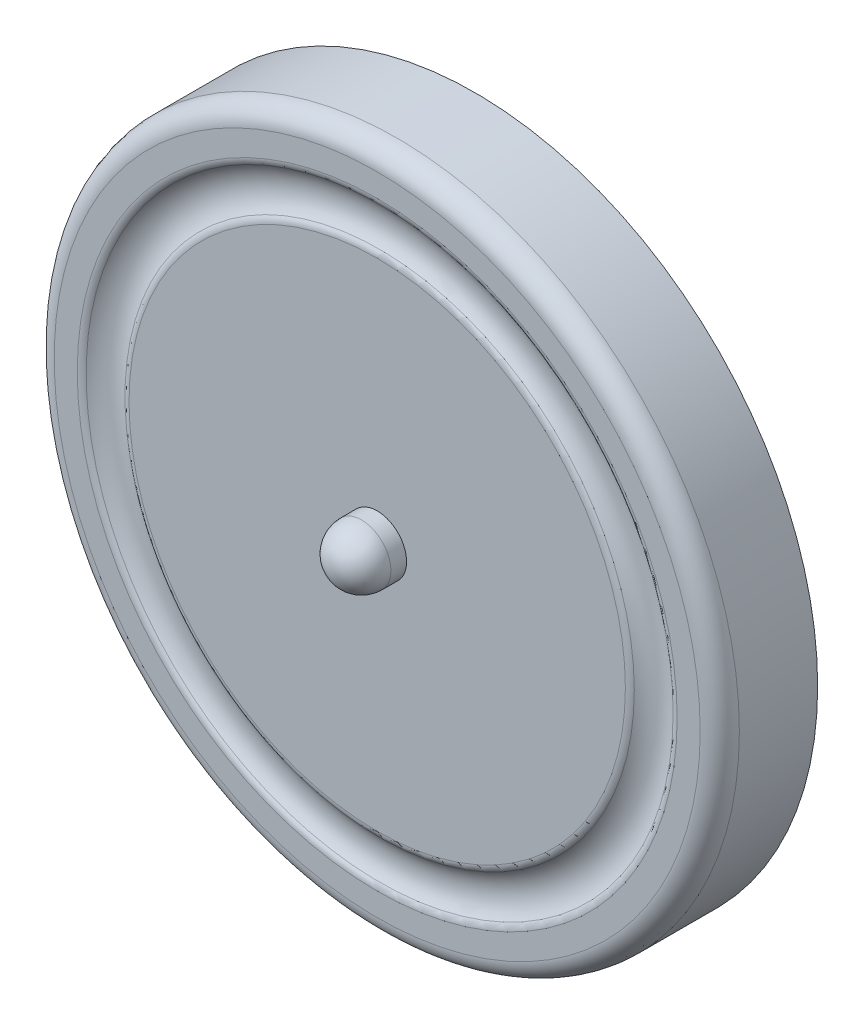
SolidWorks part; units mm, degrees
material "1.4000 (X6Cr13)"
ref_plane "Front Plane" through (0, 0, 0) normal (0, 0, 1) x (1, 0, 0)
ref_plane "Top Plane" through (0, 0, 0) normal (0, 1, 0) x (1, 0, 0)
ref_plane "Right Plane" through (0, 0, 0) normal (1, 0, 0) x (0, 0, -1)
sketch "Sketch1" plane through (0, 0, 0) normal (0, 0, 1) x (1, 0, 0)
  circle A0 centre (-121.5312, 115.619) radius 17.5
  arc A1 (-138.8054, 118.4212) -> (-107.4951, 105.1673) centre (-121.5312, 115.619) ccw construction
extrude "Boss-Extrude1" add sketch "Sketch1" along normal blind 5
ref_plane "Plane4" through (-144.5684, 61.1971, 0) normal (0.9209, -0.3898, 0) x (-0.3898, -0.9209, 0)
sketch "Sketch2" plane through (-144.5684, 61.1971, 0) normal (0.9209, -0.3898, 0) x (-0.3898, -0.9209, 0)
  line L0 (-59.097, -5.8768) -> (-59.097, 1.1833) construction
  line L1 (-59.097, -5) -> (-59.097, 0) construction
  line L2 (-59.097, -7.5) -> (-59.097, 10.5) construction
  line L3 (-41.597, 0) -> (-76.597, 0) construction
  line L4 (-59.097, 0) -> (-53.597, 0)
  line L5 (-59.097, 0) -> (-59.097, -2)
  line L6 (-59.097, -2) -> (-54.597, -2)
  line L7 (-53.597, 0) -> (-53.597, -1)
  arc A1 (-53.597, -1) -> (-54.597, -2) centre (-54.597, -1) cw
  point P14 (-53.597, -2)
  dimension "D3" = 1
  dimension "D1" = 11
  dimension "D2" = 2
revolve "Cut-Revolve1" cut sketch "Sketch2" angle 360 about L0
sketch "Sketch4" plane through (-144.5684, 61.1971, 0) normal (0.9209, -0.3898, 0) x (-0.3898, -0.9209, 0)
  line L0 (-59.097, -5) -> (-59.097, -2) construction
  line L1 (-76.597, -5) -> (-41.597, -5) construction
  line L2 (-59.097, 2.1177) -> (-59.097, -7.2354) construction
  line L3 (-59.097, 3.5) -> (-59.097, 2.5) construction
  line L4 (-54.597, -2) -> (-63.597, -2) construction
  line L7 (-59.097, -2) -> (-59.097, 3)
  arc A0 (-59.097, -2) -> (-59.097, 3) centre (-59.097, 0.5) ccw construction
  arc A1 (-59.097, -2) -> (-59.097, 3) centre (-59.097, 0.5) ccw
  dimension "D1" = 5
  dimension "D2" = 2.5
revolve "Revolve1" add sketch "Sketch4" angle 360 about L0
ref_plane "Plane5" through (0, 115.619, 0) normal (0, 1, 0) x (0, 0, 1)
sketch "Sketch5" plane through (0, 115.619, 0) normal (0, 1, 0) x (0, 0, 1)
  line L1 (5, -121.5312) -> (0, -121.5312) construction
  line L2 (5, -139.0312) -> (5, -104.0312) construction
  circle A0 centre (6, -107.5312) radius 1.5
  dimension "D2" = 3
  dimension "D1" = 14
  dimension "D3" = 1
revolve "Cut-Revolve2" cut sketch "Sketch5" angle 360 about axis through (-121.5312, 115.619, 5) along (0, 0, -1)
fillet "Fillet1" radius 1 1 edges at (-104.0312, 115.619, 5)
fillet "Fillet2" radius 0.5 2 edges at (-106.4131, 115.619, 5) (-134.4131, 115.619, 5)
sketch "Sketch6" plane through (0, 115.619, 0) normal (0, 1, 0) x (0, 0, 1)
  line L0 (0, -121.5312) -> (12.0555, -121.5312) construction
  line L1 (0, -104.0312) -> (0, -139.0312) construction
  line L2 (5.8, -120.0312) -> (4, -120.0312)
  line L3 (4, -104.0312) -> (4, -139.0312) construction
  line L4 (4, -120.0312) -> (4, -121.5312)
  line L5 (4, -121.5312) -> (7.3, -121.5312)
  line L6 (5, -138.0312) -> (5, -105.0312) construction
  arc A0 (7.3, -121.5312) -> (5.8, -120.0312) centre (5.8, -121.5312) ccw
  dimension "D1" = 3
  dimension "D2" = 0.8
revolve "Revolve2" add sketch "Sketch6" angle 360 about L0
